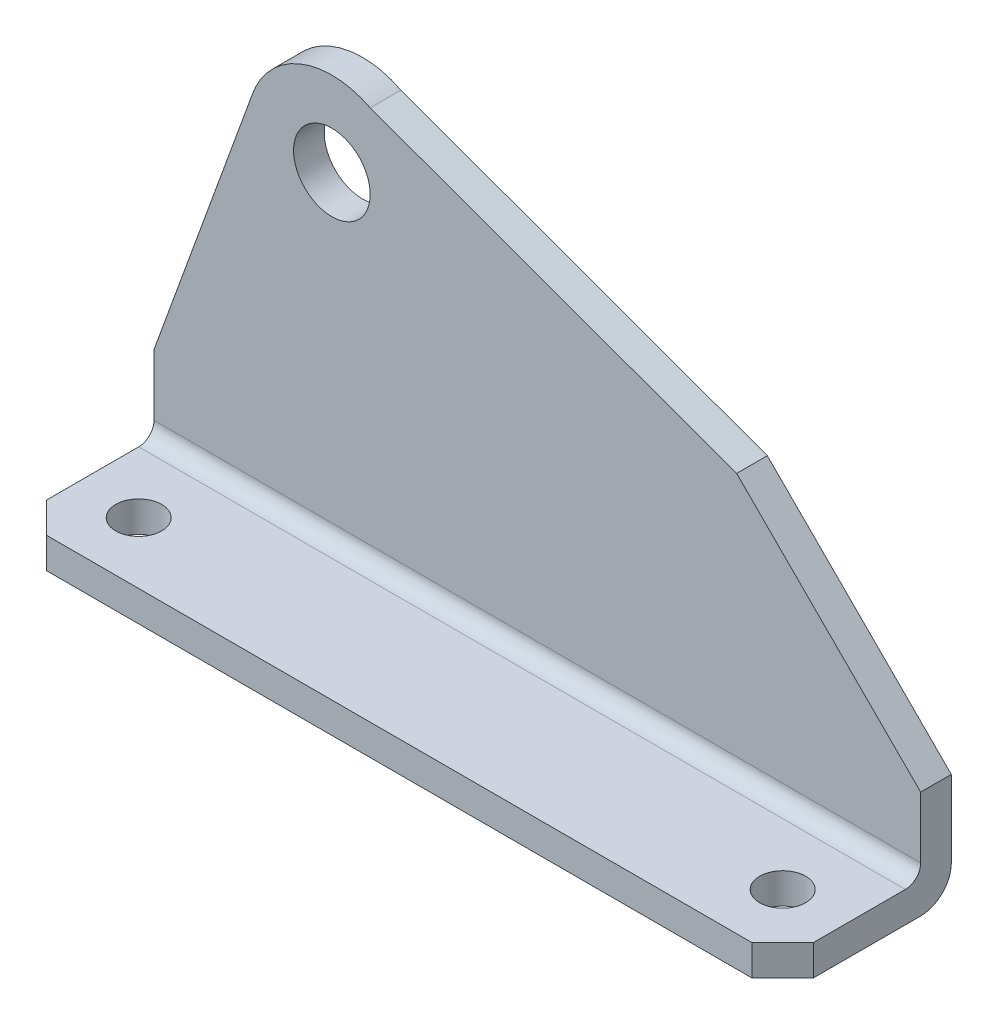
from build123d import *

# Parameters (mm, degrees)
SKETCH1_W           = 250
SKETCH1_H           = 181
BOSS_EXTRUDE1_DEPTH = 10
SKETCH2_OUTSIDE_W   = 313.762
SKETCH2_OUTSIDE_H   = 244.762
CUT_EXTRUDE1_DEPTH  = 10
SKETCH3_R           = 12.5
CUT_EXTRUDE2_DEPTH  = 10
SKETCH6_W           = 250
SKETCH6_H           = 10
BOSS_EXTRUDE3_DEPTH = 45
FILLET3_R           = 5
FILLET4_R           = 10
SKETCH7_R           = 7.5
CUT_EXTRUDE4_DEPTH  = 45
CHAMFER2_SIZE       = 10


with BuildPart() as part:
    # Sketch1 → Boss-Extrude1 (new body)
    with BuildSketch(Plane.XY):
        Rectangle(SKETCH1_W, SKETCH1_H)
    extrude(amount=BOSS_EXTRUDE1_DEPTH)

    # Sketch2 outside → Cut-Extrude1 (cut)
    with BuildSketch(Plane.XY.offset(10)):
        Rectangle(SKETCH2_OUTSIDE_W, SKETCH2_OUTSIDE_H)
        with BuildLine():
            Line((-125, -55.5), (-93.159896838, 31.97996447))
            ThreePointArc((-93.159896838, 31.97996447), (-77.523014584, 48.907010136), (-54.496896373, 47.993313367))
            Line((-54.496896373, 47.993313367), (65, 4.5))
            Line((65, 4.5), (125, -55.5))
            Line((125, -55.5), (125, -90.5))
            Line((125, -90.5), (-125, -90.5))
            Line((-125, -90.5), (-125, -55.5))
        make_face(mode=Mode.SUBTRACT)
    extrude(amount=-CUT_EXTRUDE1_DEPTH, mode=Mode.SUBTRACT)

    # Sketch3 → Cut-Extrude2 (cut)
    with BuildSketch(Plane.XY.offset(10)):
        with Locations((-67, 23.5)):
            Circle(SKETCH3_R)
    extrude(amount=-CUT_EXTRUDE2_DEPTH, mode=Mode.SUBTRACT)

    # Sketch6 → Boss-Extrude3 (add)
    with BuildSketch(Plane.XY.offset(10)):
        with Locations((0, -85.5)):
            Rectangle(SKETCH6_W, SKETCH6_H)
    extrude(amount=BOSS_EXTRUDE3_DEPTH)

    # Fillet3
    fillet3_edges = [part.edges().sort_by_distance(p)[0] for p in [
        (0, -80.5, 10),
    ]]
    fillet(fillet3_edges, radius=FILLET3_R)

    # Fillet4
    fillet4_edges = [part.edges().sort_by_distance(p)[0] for p in [
        (0, -90.5, 0),
    ]]
    fillet(fillet4_edges, radius=FILLET4_R)

    # Sketch7 → Cut-Extrude4 (cut)
    with BuildSketch(Plane.XZ.offset(90.5)):
        with Locations((-105, 35)):
            Circle(SKETCH7_R)
        with Locations((105, 35)):
            Circle(SKETCH7_R)
    extrude(amount=-CUT_EXTRUDE4_DEPTH, mode=Mode.SUBTRACT)

    # Chamfer2
    chamfer2_edges = [part.edges().sort_by_distance(p)[0] for p in [
        (-125, -85.5, 55),
        (125, -85.5, 55),
    ]]
    chamfer(chamfer2_edges, length=CHAMFER2_SIZE)


solid = part.part
